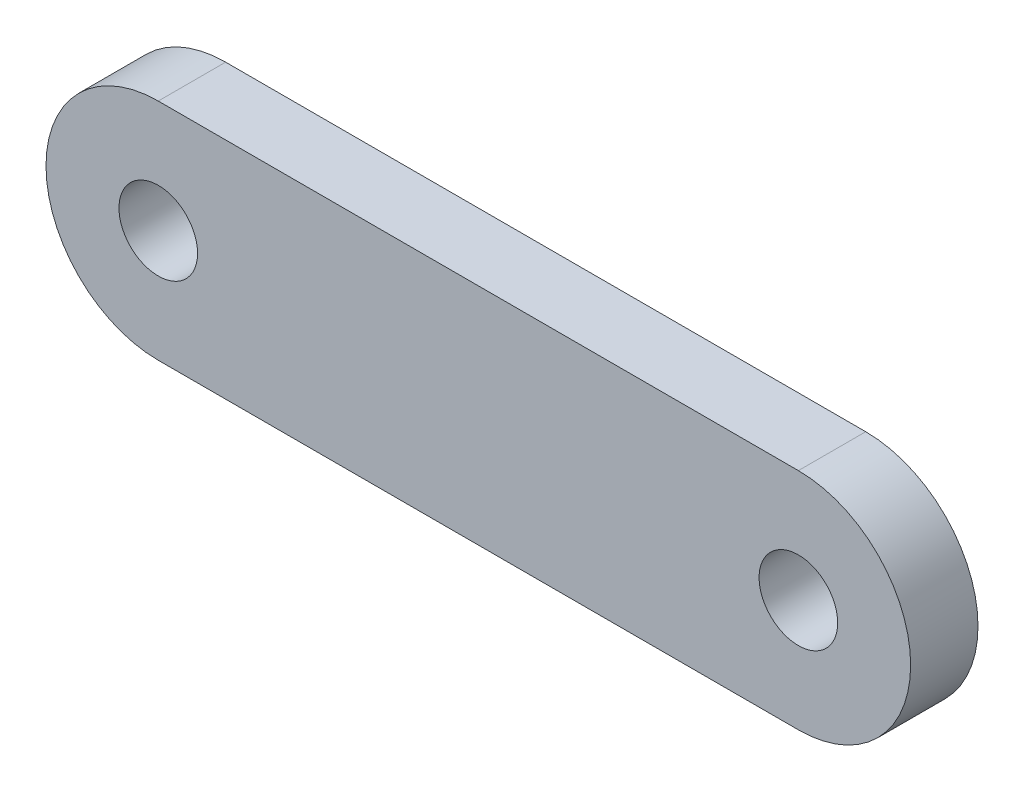
from build123d import *

# Parameters (mm, degrees)
BOSS_EXTRUDE1_DEPTH = 6
SKETCH2_R           = 3.5
CUT_EXTRUDE1_DEPTH  = 95


with BuildPart() as part:
    # Sketch1 → Boss-Extrude1 (new body)
    with BuildSketch(Plane.XY):
        with BuildLine():
            Line((0, 10), (57.02, 10))
            ThreePointArc((57.02, 10), (67.02, 0), (57.02, -10))
            Line((57.02, -10), (0, -10))
            ThreePointArc((0, -10), (-10, 0), (0, 10))
        make_face()
    extrude(amount=BOSS_EXTRUDE1_DEPTH)

    # Sketch2 → Cut-Extrude1 (cut)
    with BuildSketch(Plane.XY.offset(6)):
        Circle(SKETCH2_R)
        with Locations((57.02, 0)):
            Circle(SKETCH2_R)
    extrude(amount=-CUT_EXTRUDE1_DEPTH, mode=Mode.SUBTRACT)


solid = part.part
